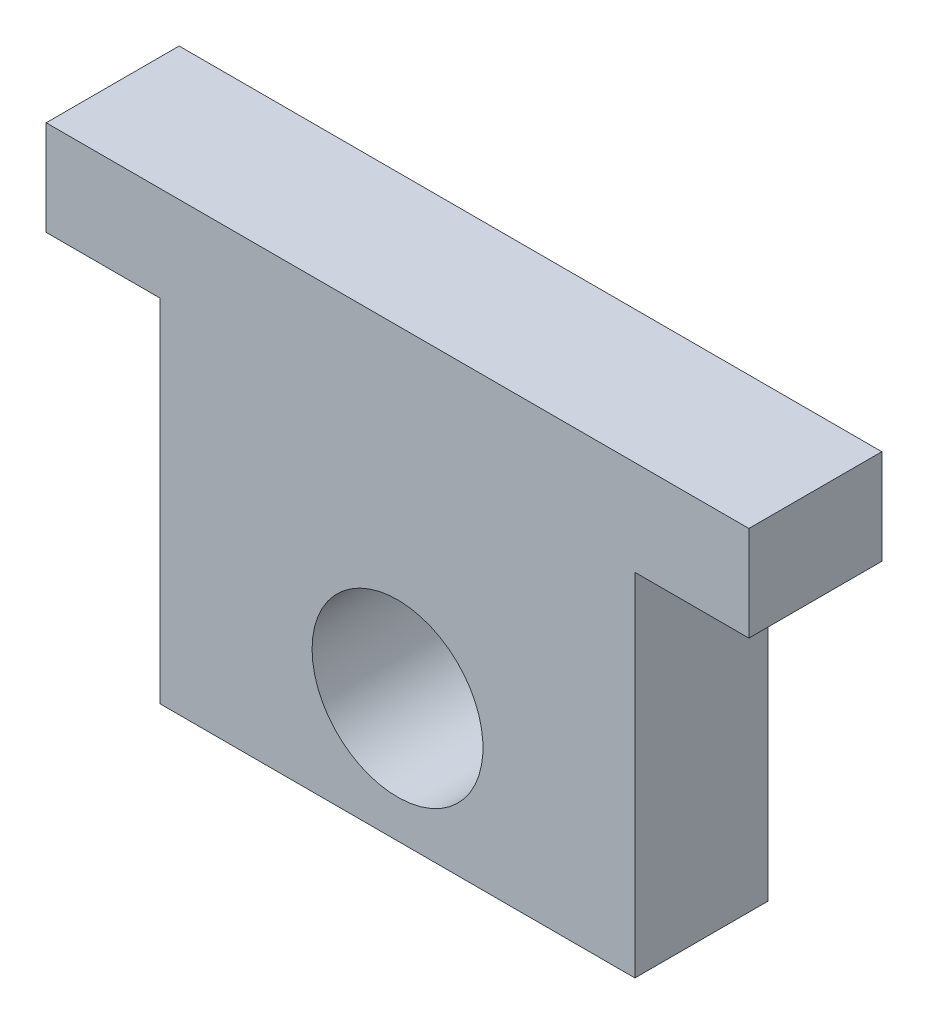
from build123d import *

# Parameters (mm, degrees)
SKETCH_1_W          = 50
SKETCH_1_H          = 47
EXTRUDE_1_DEPTH     = 7
CUT_EXTRUDE_1_REACH = 39.057
SKETCH_2_R          = 9
SKETCH_4_W          = 12
SKETCH_4_H          = 14
EXTRUDE_2_DEPTH     = 10


with BuildPart() as part:
    # 草图1 → 凸台-拉伸1 (new, symmetric)
    with BuildSketch(Plane.XY):
        Rectangle(SKETCH_1_W, SKETCH_1_H)
    extrude(amount=EXTRUDE_1_DEPTH, both=True)

    # 草图2 → 切除-拉伸1 (cut, up to next)
    with BuildSketch(Plane(origin=(0, 0, -7), x_dir=(-1, 0, 0), z_dir=(0, 0, -1)), mode=Mode.PRIVATE) as cut_extrude_1_sk1:
        with Locations((0, -10.5)):
            Circle(SKETCH_2_R)
    cut_extrude_1_tool1 = extrude(cut_extrude_1_sk1.sketch, amount=-CUT_EXTRUDE_1_REACH, mode=Mode.PRIVATE) & part.part
    add(cut_extrude_1_tool1.solids().sort_by_distance((0, -10.5, -7))[0], mode=Mode.SUBTRACT)

    # 草图4 → 凸台-拉伸2 (add)
    with BuildSketch(Plane(origin=(0, 23.5, 0), x_dir=(1, 0, 0), z_dir=(0, 1, 0))):
        with Locations((31, 0)):
            Rectangle(SKETCH_4_W, SKETCH_4_H)
        with Locations((-31, 0)):
            Rectangle(SKETCH_4_W, SKETCH_4_H)
    extrude(amount=-EXTRUDE_2_DEPTH)


solid = part.part
